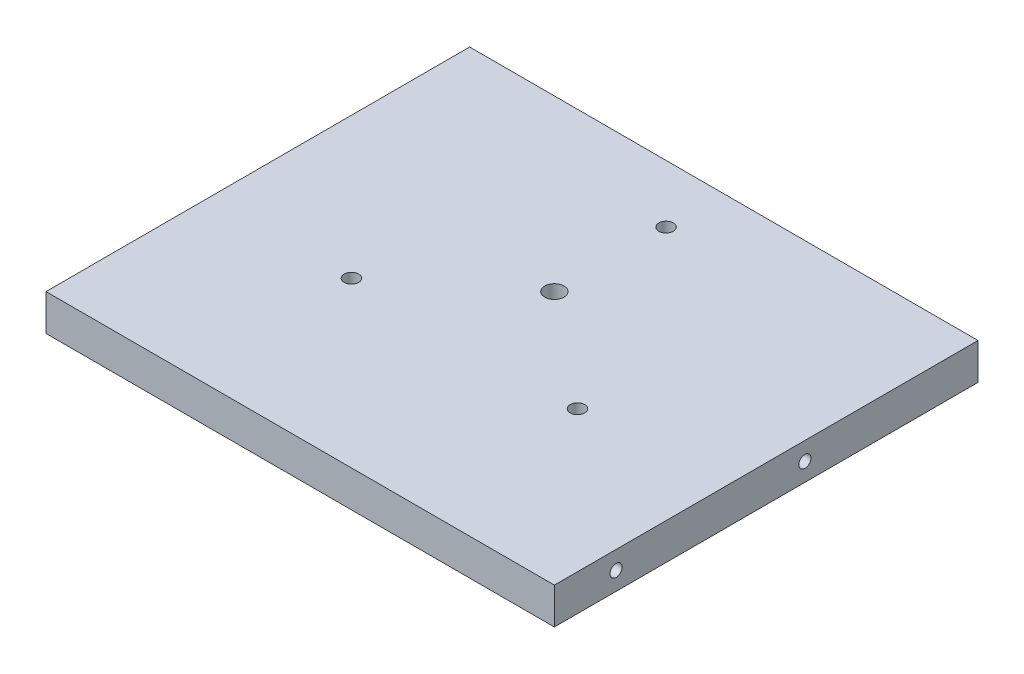
from build123d import *

# Parameters (mm, degrees)
SKETCH1_W                 = 210
SKETCH1_H                 = 175
BOSS_EXTRUDE1_DEPTH       = 15
SKETCH3_R                 = 5
SKETCH3_R_2               = 3
CUT_EXTRUDE1_DEPTH        = 6
CUT_EXTRUDE2_REACH        = 139.5
SKETCH3_3_R               = 3
M6X1_0_TAPPED_HOLE1_D     = 5
M6X1_0_TAPPED_HOLE1_DEPTH = 15
M6X1_0_TAPPED_HOLE1_TIP   = 1.502151548
M6X1_0_TAPPED_HOLE2_D     = 5
M6X1_0_TAPPED_HOLE2_DEPTH = 15
M6X1_0_TAPPED_HOLE2_TIP   = 1.502151548
SKETCH8_R                 = 6.5
SKETCH8_R_2               = 4
CUT_EXTRUDE3_DEPTH        = 8
CUT_EXTRUDE4_REACH        = 139.5
SKETCH8_3_R               = 4


with BuildPart() as part:
    # Sketch1 → Boss-Extrude1 (new body)
    with BuildSketch(Plane(origin=(0, 0, 0), x_dir=(1, 0, 0), z_dir=(0, 1, 0))):
        Rectangle(SKETCH1_W, SKETCH1_H)
    extrude(amount=BOSS_EXTRUDE1_DEPTH)

    # Sketch3 → Cut-Extrude1 (cut)
    # profile 1 of 3: a face of its own
    with BuildSketch(Plane.XZ):
        with Locations(Location((-46.687978245, 19.63800195, 0), (0, 0, 270))):
            Circle(SKETCH3_R)
        with Locations(Location((-46.687978245, 19.63800195, 0), (0, 0, 270))):
            Circle(SKETCH3_R_2, mode=Mode.SUBTRACT)
    # profile 2 of 3: a face of its own
    with BuildSketch(Plane.XZ):
        with Locations(Location((46.687978245, 19.63800195, 0), (0, 0, 270))):
            Circle(SKETCH3_R)
        with Locations(Location((46.687978245, 19.63800195, 0), (0, 0, 270))):
            Circle(SKETCH3_R_2, mode=Mode.SUBTRACT)
    # profile 3 of 3: a face of its own
    with BuildSketch(Plane.XZ):
        with Locations(Location((0, -63.6274596, 0), (0, 0, 270))):
            Circle(SKETCH3_R)
        with Locations(Location((0, -63.6274596, 0), (0, 0, 270))):
            Circle(SKETCH3_R_2, mode=Mode.SUBTRACT)
    extrude(amount=-CUT_EXTRUDE1_DEPTH, mode=Mode.SUBTRACT)

    # Sketch3<3> → Cut-Extrude2 (cut, up to next)
    with BuildSketch(Plane.XZ, mode=Mode.PRIVATE) as cut_extrude2_sk1:
        with Locations(Location((-46.687978245, 19.63800195, 0), (0, 0, 270))):
            Circle(SKETCH3_3_R)
    cut_extrude2_tool1 = extrude(cut_extrude2_sk1.sketch, amount=-CUT_EXTRUDE2_REACH, mode=Mode.PRIVATE) & part.part
    # Sketch3<3> → Cut-Extrude2 (cut, up to next)
    with BuildSketch(Plane.XZ, mode=Mode.PRIVATE) as cut_extrude2_sk2:
        with Locations(Location((46.687978245, 19.63800195, 0), (0, 0, 270))):
            Circle(SKETCH3_3_R)
    cut_extrude2_tool2 = extrude(cut_extrude2_sk2.sketch, amount=-CUT_EXTRUDE2_REACH, mode=Mode.PRIVATE) & part.part
    # Sketch3<3> → Cut-Extrude2 (cut, up to next)
    with BuildSketch(Plane.XZ, mode=Mode.PRIVATE) as cut_extrude2_sk3:
        with Locations(Location((0, -63.6274596, 0), (0, 0, 270))):
            Circle(SKETCH3_3_R)
    cut_extrude2_tool3 = extrude(cut_extrude2_sk3.sketch, amount=-CUT_EXTRUDE2_REACH, mode=Mode.PRIVATE) & part.part
    add(cut_extrude2_tool1.solids().sort_by_distance((-46.687978, 0, 19.638002))[0], mode=Mode.SUBTRACT)
    add(cut_extrude2_tool2.solids().sort_by_distance((46.687978, 0, 19.638002))[0], mode=Mode.SUBTRACT)
    add(cut_extrude2_tool3.solids().sort_by_distance((0, 0, -63.62746))[0], mode=Mode.SUBTRACT)

    # M6x1.0 Tapped Hole1
    with Locations(Plane(origin=(105, 7.5, -16), x_dir=(0, 0, 1), z_dir=(1, 0, 0))):
        with Locations((0, 0), (78, 0)):
            Hole(M6X1_0_TAPPED_HOLE1_D / 2, depth=M6X1_0_TAPPED_HOLE1_DEPTH)
            with Locations((0, 0, -(M6X1_0_TAPPED_HOLE1_DEPTH + M6X1_0_TAPPED_HOLE1_TIP / 2))):  # 118° drill point
                Cone(0, M6X1_0_TAPPED_HOLE1_D / 2, M6X1_0_TAPPED_HOLE1_TIP, mode=Mode.SUBTRACT)

    # M6x1.0 Tapped Hole2
    with Locations(Plane(origin=(80, 7.5, -87.5), x_dir=(-1, 0, 0), z_dir=(0, 0, -1))):
        with Locations((0, 0), (80, 0), (160, 0)):
            Hole(M6X1_0_TAPPED_HOLE2_D / 2, depth=M6X1_0_TAPPED_HOLE2_DEPTH)
            with Locations((0, 0, -(M6X1_0_TAPPED_HOLE2_DEPTH + M6X1_0_TAPPED_HOLE2_TIP / 2))):  # 118° drill point
                Cone(0, M6X1_0_TAPPED_HOLE2_D / 2, M6X1_0_TAPPED_HOLE2_TIP, mode=Mode.SUBTRACT)

    # Sketch8 → Cut-Extrude3 (cut)
    with BuildSketch(Plane(origin=(0, 0, 0), x_dir=(-1, 0, 0), z_dir=(0, -1, 0))):
        with Locations(Location((0, 17.5, 0), (0, 0, 90))):
            Circle(SKETCH8_R)
        with Locations(Location((0, 17.5, 0), (0, 0, 90))):
            Circle(SKETCH8_R_2, mode=Mode.SUBTRACT)
    extrude(amount=-CUT_EXTRUDE3_DEPTH, mode=Mode.SUBTRACT)

    # Sketch8<3> → Cut-Extrude4 (cut, up to next)
    with BuildSketch(Plane(origin=(0, 0, 0), x_dir=(-1, 0, 0), z_dir=(0, -1, 0)), mode=Mode.PRIVATE) as cut_extrude4_sk1:
        with Locations(Location((0, 17.5, 0), (0, 0, 90))):
            Circle(SKETCH8_3_R)
    cut_extrude4_tool1 = extrude(cut_extrude4_sk1.sketch, amount=-CUT_EXTRUDE4_REACH, mode=Mode.PRIVATE) & part.part
    add(cut_extrude4_tool1.solids().sort_by_distance((0, 0, -17.5))[0], mode=Mode.SUBTRACT)


solid = part.part
